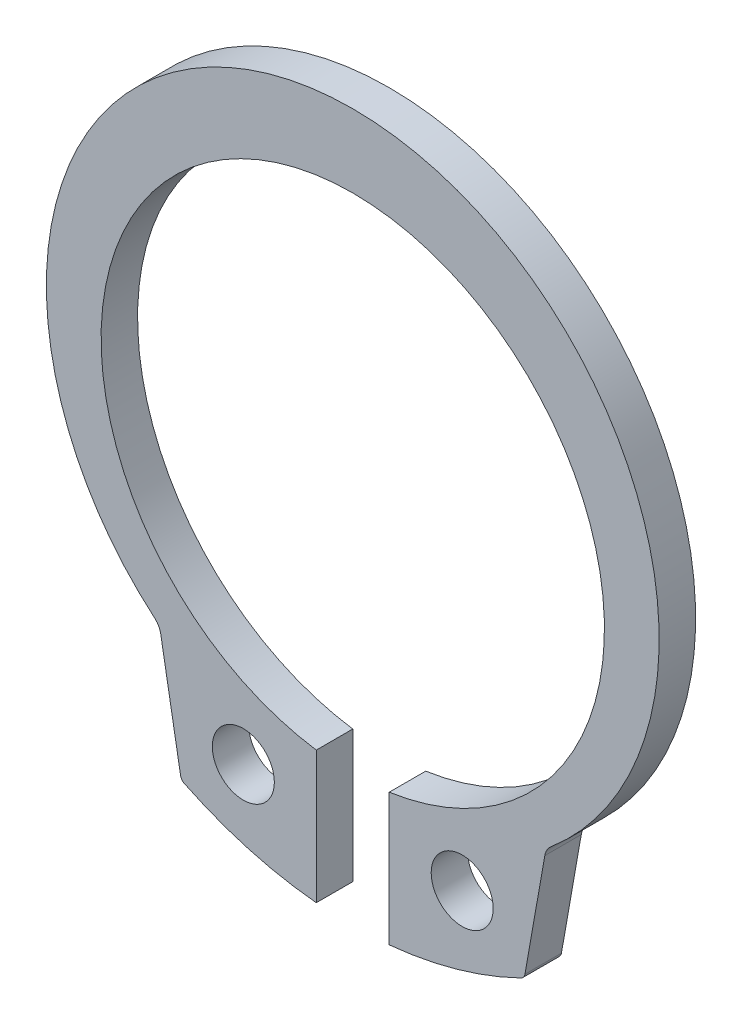
from build123d import *

# Parameters (mm, degrees)
SKETCH1_R  = 0.85
BODY_DEPTH = 1
FILLET1_R  = 0.2
FILLET2_R  = 0.5


with BuildPart() as part:
    # Sketch1 → Body (new body)
    with BuildSketch(Plane.XY):
        with BuildLine():
            Line((-1, -7.327151675), (-1, -10.95227248))
            ThreePointArc((-1, -10.95227248), (-2.900753364, -10.591364126), (-4.703022713, -9.887841997))
            Line((-4.703022713, -9.887841997), (-5.296977287, -6.519358222))
            ThreePointArc((-5.296977287, -6.519358222), (0, 8.4), (5.296977287, -6.519358222))
            Line((5.296977287, -6.519358222), (4.703022713, -9.887841997))
            ThreePointArc((4.703022713, -9.887841997), (2.900753364, -10.591364126), (1, -10.95227248))
            Line((1, -10.95227248), (1, -7.327151675))
            ThreePointArc((1, -7.327151675), (0, 6.4), (-1, -7.327151675))
        make_face()
        with Locations(Location((3, -8.666394553, 0), (0, 0, 180))):
            Circle(SKETCH1_R, mode=Mode.SUBTRACT)
        with Locations((-3, -8.666394553)):
            Circle(SKETCH1_R, mode=Mode.SUBTRACT)
    extrude(amount=-BODY_DEPTH)

    # Fillet1
    fillet1_edges = [part.edges().sort_by_distance(p)[0] for p in [
        (-4.703022713, -9.887841997, -0.5),
        (4.703022713, -9.887841997, -0.5),
    ]]
    fillet(fillet1_edges, radius=FILLET1_R)

    # Fillet2
    fillet2_edges = [part.edges().sort_by_distance(p)[0] for p in [
        (-5.296977287, -6.519358222, -0.5),
        (5.296977287, -6.519358222, -0.5),
    ]]
    fillet(fillet2_edges, radius=FILLET2_R)


solid = part.part
